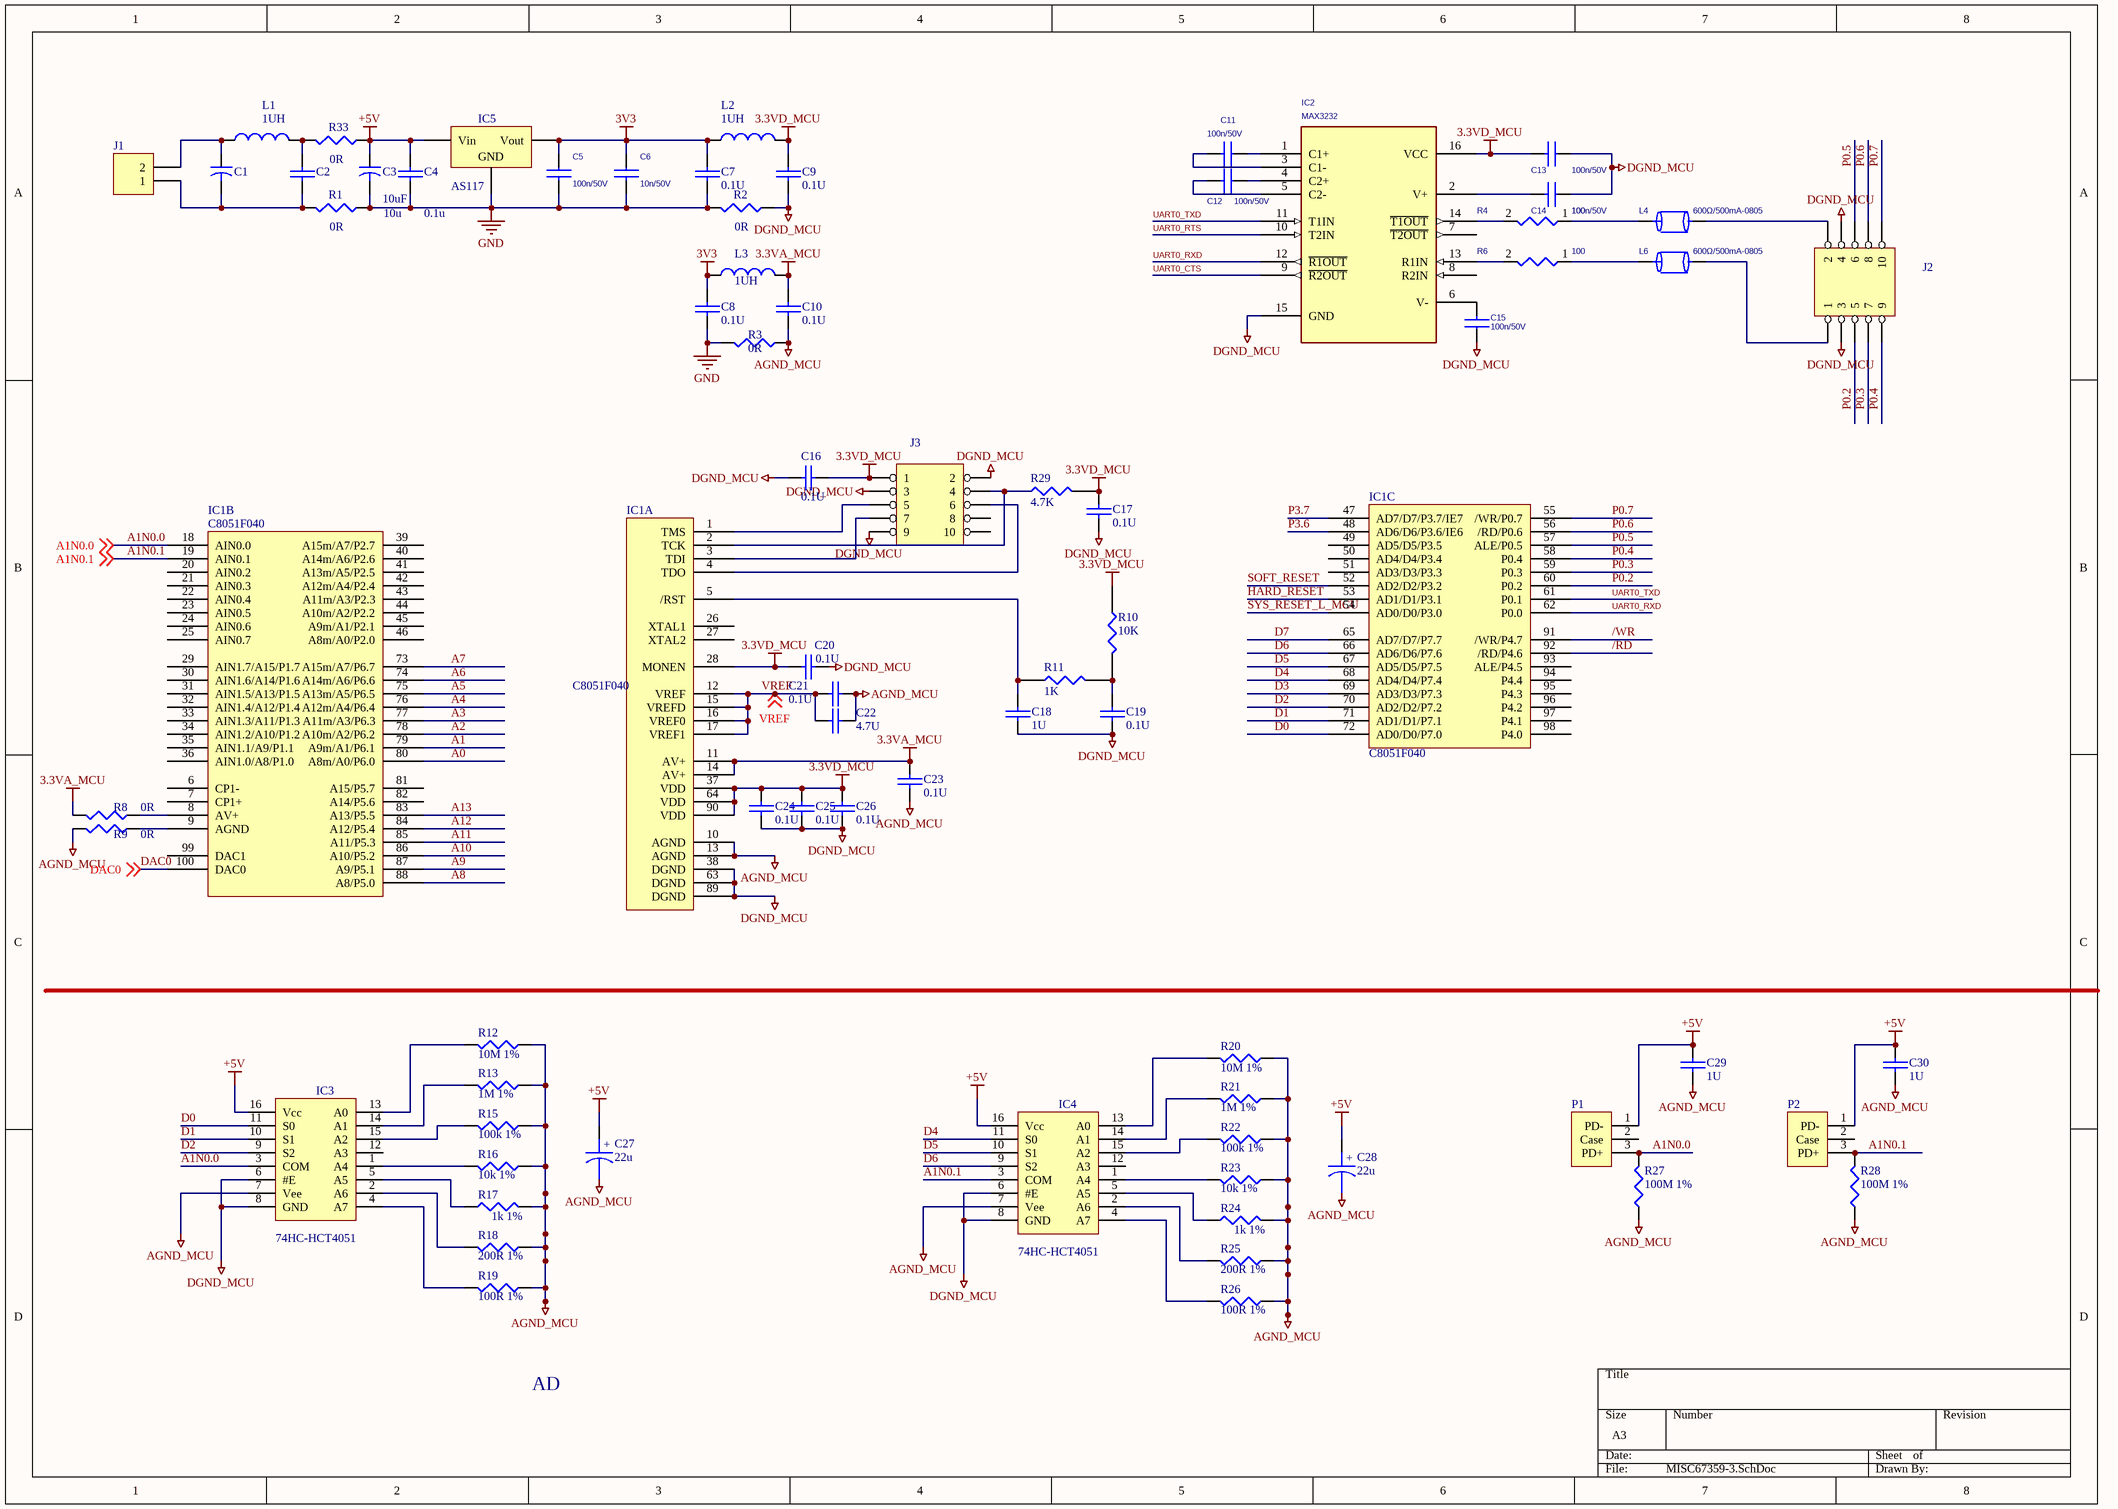
[diagram p0: MISC67359-3.SchDoc]
# Altium project MISC67359-2.PrjPcb
1 sheet, 72 parts. Net scope: global (net labels, ports and power ports of the same name join across sheets).
Board file: MISC67359.PcbDoc

## Sheet MISC67359-3.SchDoc
size A3; SheetNumber: 10; SheetTotal: 14

### Parts
C1  (no value)  [CAPC3216N]
C2  (no value)  [CAPC3216N]
C3  10u  value 10uF  [CAPC2012N]
C4  0.1u  [0603]
C5  100n/50V  [0603]
C6  10n/50V  [0603]
C7  0.1U  [0603]
C8  0.1U  [0603]
C9  0.1U  [0603]
C10  0.1U  [0603]
C11  100n/50V  [0603]
C12  100n/50V  [0603]
C13  100n/50V  [0603]
C14  100n/50V  [0603]
C15  100n/50V  [0603]
C16  0.1U  [0603]
C17  0.1U  [0603]
C18  1U  [0603]
C19  0.1U  [0603]
C20  0.1U  [0603]
C21  0.1U  [0603]
C22  4.7U  [0603]
C23  0.1U  [0603]
C24  0.1U  [0603]
C25  0.1U  [0603]
C26  0.1U  [0603]
C27  22u  [3528]
C28  22u  [3528]
C29  1U  [0603]
C30  1U  [0603]
IC1  C8051F040  [TQFP100]  (parts A,B,C of 3)
IC2  MAX3232  [SOIC127P600-16N]
IC3  74HC-HCT4051  [SOIC16]
IC4  74HC-HCT4051  [SOIC16]
IC5  AS117  [SOT89L]
J1  (no value)  [MKDS3_2RMI]
J2  (no value)  [FKV10SN]
J3  (no value)  [FKV10SN]
L1  1UH  [0805]
L2  1UH  [0805]
L3  1UH  [0805]
L4  600Ω/500mA-0805  [0805]
L6  600Ω/500mA-0805  [0805]
P1  (no value)  [E3]
P2  (no value)  [E3]
R1  0R  [6-0805_N]
R2  0R  [6-0805_N]
R3  0R  [6-0805_N]
R4  100  [0603]
R6  100  [0603]
R8  0R  [0603]
R9  0R  [0603]
R10  10K  [0603]
R11  1K  [0603]
R12  10M 1%  [0603]
R13  1M 1%  [0603]
R15  100k 1%  [0603]
R16  10k 1%  [0603]
R17  1k 1%  [0603]
R18  200R 1%  [0603]
R19  100R 1%  [0603]
R20  10M 1%  [0603]
R21  1M 1%  [0603]
R22  100k 1%  [0603]
R23  10k 1%  [0603]
R24  1k 1%  [0603]
R25  200R 1%  [0603]
R26  100R 1%  [0603]
R27  100M 1%  [0603]
R28  100M 1%  [0603]
R29  4.7K  [0603]
R33  0R  [6-0805_N]

### Nets
3.3VA_MCU: C10.1 C23.2 IC1.11(AV+) IC1.14(AV+) L3.1 R8.1
3.3VD_MCU: C9.1 C13.2 C16.2 C17.1 C20.2 C24.2 C25.2 C26.2 IC1.28(MONEN) IC1.37(VDD) IC1.64(VDD) IC1.90(VDD) IC2.16(VCC) J3.1 L2.2 R10.2 R29.1
3V3: C5.1 C6.1 C7.2 C8.2 IC5.2(Vout) L2.1 L3.2
+5V: C3.1 C4.1 C27.1 C28.1 C29.2 C30.2 IC3.16(Vcc) IC4.16(Vcc) IC5.3(Vin) P1.1(PD-) P2.1(PD-) R33.2
AGND_MCU: C10.2 C21.1 C22.1 C23.1 C27.2 C28.2 C29.1 C30.1 IC1.10(AGND) IC1.13(AGND) IC3.7(Vee) IC4.7(Vee) R3.2 R9.1 R12.1 R13.1 R15.1 R16.1 R17.2 R18.1 R19.1 R20.1 R21.1 R22.1 R23.1 R24.2 R25.1 R26.1 R27.1 R28.1
DGND_MCU: C9.2 C13.1 C14.1 C15.1 C16.1 C17.2 C18.1 C19.1 C20.1 C24.1 C25.1 C26.1 IC1.38(DGND) IC1.63(DGND) IC1.89(DGND) IC2.15(GND) IC3.6(#E) IC3.8(GND) IC4.6(#E) IC4.8(GND) J2.3 J2.4 J3.2 J3.3 J3.9 R2.2
GND: C3.2 C4.2 C5.2 C6.2 C7.1 C8.1 IC5.1(GND) R1.2 R2.1 R3.1
/RD: IC1.92(/RD/P4.6)
/WR: IC1.91(/WR/P4.7)
A0: IC1.80(A8m/A0/P6.0)
A1: IC1.79(A9m/A1/P6.1)
A1N0.0: IC1.18(AIN0.0) IC3.3(COM) P1.3(PD+) R27.2 ; off-sheet A1N0.0
A1N0.1: IC1.19(AIN0.1) IC4.3(COM) P2.3(PD+) R28.2 ; off-sheet A1N0.1
A2: IC1.78(A10m/A2/P6.2)
A3: IC1.77(A11m/A3/P6.3)
A4: IC1.76(A12m/A4/P6.4)
A5: IC1.75(A13m/A5/P6.5)
A6: IC1.74(A14m/A6/P6.6)
A7: IC1.73(A15m/A7/P6.7)
A8: IC1.88(A8/P5.0)
A9: IC1.87(A9/P5.1)
A10: IC1.86(A10/P5.2)
A11: IC1.85(A11/P5.3)
A12: IC1.84(A12/P5.4)
A13: IC1.83(A13/P5.5)
D0: IC1.72(AD0/D0/P7.0) IC3.11(S0)
D1: IC1.71(AD1/D1/P7.1) IC3.10(S1)
D2: IC1.70(AD2/D2/P7.2) IC3.9(S2)
D3: IC1.69(AD3/D3/P7.3)
D4: IC1.68(AD4/D4/P7.4) IC4.11(S0)
D5: IC1.67(AD5/D5/P7.5) IC4.10(S1)
D6: IC1.66(AD6/D6/P7.6) IC4.9(S2)
D7: IC1.65(AD7/D7/P7.7)
DAC0: IC1.100(DAC0) ; off-sheet DAC0
HARD_RESET: IC1.53(AD1/D1/P3.1)
P0.2: IC1.60(P0.2) J2.5
P0.3: IC1.59(P0.3) J2.7
P0.4: IC1.58(P0.4) J2.9
P0.5: IC1.57(ALE/P0.5) J2.6
P0.6: IC1.56(/RD/P0.6) J2.8
P0.7: IC1.55(/WR/P0.7) J2.10
P3.6: IC1.48(AD6/D6/P3.6/IE6)
P3.7: IC1.47(AD7/D7/P3.7/IE7)
SOFT_RESET: IC1.52(AD2/D2/P3.2)
SYS_RESET_L_MCU: IC1.54(AD0/D0/P3.0)
UART0_CTS: IC2.9(~{R2OUT})
UART0_RTS: IC2.10(T2IN)
UART0_RXD: IC1.62(P0.0) IC2.12(~{R1OUT})
UART0_TXD: IC1.61(P0.1) IC2.11(T1IN)
VREF: C21.2 C22.2 IC1.12(VREF) IC1.15(VREFD) IC1.16(VREF0) IC1.17(VREF1) ; off-sheet VREF
NetC1_1: C1.1 J1.2 L1.1
NetC1_2: C1.2 C2.2 J1.1 R1.1
NetC2_1: C2.1 L1.2 R33.1
NetC11_1: C11.1 IC2.1(C1+)
NetC11_2: C11.2 IC2.3(C1-)
NetC12_1: C12.1 IC2.4(C2+)
NetC12_2: C12.2 IC2.5(C2-)
NetC14_2: C14.2 IC2.2(V+)
NetC15_2: C15.2 IC2.6(V-)
NetC18_2: C18.2 IC1.5(/RST) R11.2
NetC19_2: C19.2 R10.1 R11.1
NetIC1_1: IC1.1(TMS) J3.5
NetIC1_2: IC1.2(TCK) J3.4 R29.2
NetIC1_3: IC1.3(TDI) J3.7
NetIC1_4: IC1.4(TDO) J3.6
NetIC1_8: IC1.8(AV+) R8.2
NetIC1_9: IC1.9(AGND) R9.2
NetIC2_13: IC2.13(R1IN) R6.2
NetIC2_14: IC2.14(~{T1OUT}) R4.2
NetIC3_1: IC3.1(A4) R16.2
NetIC3_2: IC3.2(A6) R18.2
NetIC3_4: IC3.4(A7) R19.2
NetIC3_5: IC3.5(A5) R17.1
NetIC3_13: IC3.13(A0) R12.2
NetIC3_14: IC3.14(A1) R13.2
NetIC3_15: IC3.15(A2) R15.2
NetIC4_1: IC4.1(A4) R23.2
NetIC4_2: IC4.2(A6) R25.2
NetIC4_4: IC4.4(A7) R26.2
NetIC4_5: IC4.5(A5) R24.1
NetIC4_13: IC4.13(A0) R20.2
NetIC4_14: IC4.14(A1) R21.2
NetIC4_15: IC4.15(A2) R22.2
NetJ2_1: J2.1 L6.2
NetJ2_2: J2.2 L4.2
NetL4_1: L4.1 R4.1
NetL6_1: L6.1 R6.1

Not connected (* = marked no-connect by the designer): IC1 6(CP1-) 7(CP1+) 20(AIN0.2) 21(AIN0.3) 22(AIN0.4) 23(AIN0.5) 24(AIN0.6) 25(AIN0.7) 26(XTAL1) 27(XTAL2) 29(AIN1.7/A15/P1.7) 30(AIN1.6/A14/P1.6) 31(AIN1.5/A13/P1.5) 32(AIN1.4/A12/P1.4) 33(AIN1.3/A11/P1.3) 34(AIN1.2/A10/P1.2) 35(AIN1.1/A9/P1.1) 36(AIN1.0/A8/P1.0) 39(A15m/A7/P2.7) 40(A14m/A6/P2.6) 41(A13m/A5/P2.5) 42(A12m/A4/P2.4) 43(A11m/A3/P2.3) 44(A10m/A2/P2.2) 45(A9m/A1/P2.1) 46(A8m/A0/P2.0) 49(AD5/D5/P3.5) 50(AD4/D4/P3.4) 51(AD3/D3/P3.3) 81(A15/P5.7) 82(A14/P5.6) 93(ALE/P4.5) 94(P4.4) 95(P4.3) 96(P4.2) 97(P4.1) 98(P4.0) 99(DAC1); IC2 7(~{T2OUT}) 8(R2IN); IC3 12(A3); IC4 12(A3); J3 8 10; P1 2(Case); P2 2(Case)

### Notes on the sheet
- AD

### Library data of the parts
C1 = Cap2: Capacitor; Value: 10uF; Published: 23-Sep-2002; PackageReference: CAPR5-4X5; PackageDescription: Capacitor; 2 Leads; Publisher: Altium Limited
C2 C4 C7-C10 C16-C26 C29 C30 = CAP: Capacitor
C3 = Cap2: Capacitor; Published: 23-Sep-2002; PackageReference: CAPR5-4X5; PackageDescription: Capacitor; 2 Leads; Publisher: Altium Limited
C5 C6 C11-C15 = CAPACITOR NON-POL
C27 C28 = CAPACITOR POL
IC1 = C8051F020
IC3 IC4 = CD54HC4051
IC5 = Volt Reg: Voltage Regulator; Published: 24-Mar-1999; LatestRevisionDate: 17-Jul-2002; LatestRevisionNote: Re-released for DXP Platform.; PackageReference: D2PAK; Code_JEDEC: SMD-220; Publisher: Altium Limited
J1 = Header 2: Header, 2-Pin; LatestRevisionDate: 17-Jul-2002; LatestRevisionNote: Re-released for DXP Platform.; Publisher: Altium Limited
J2 J3 = HEADER 5X2
L1-L3 = INDUCTOR: Text Field1: 10; Text Field2: 40
L4 L6 = BEAD: Part Number: 20.43.10.0007.01; 替: 1; 厂: TDK; 规: TDK_MMZ2012S601AT000; Value1: 600Ω/500mA-0805; 物: 0805
P1 P2 = MHDR1X3
R1-R3 R8 R9 R33 = RES: Resistor; TC: *
R4 R6 = SMDRXX_2: COMPHEIGHT: 0.000; MEMORY: NO; COMPGROUP: 0; COMPROT: 90; COMPLOC: [2325.000,2475.000]; COMPSIDE: TOP; DECOUPLER: NO; COMPKEY: NO; COMPLOCKED: NO; COMPFIXED: NO
R10-R13 R15-R29 = RES1